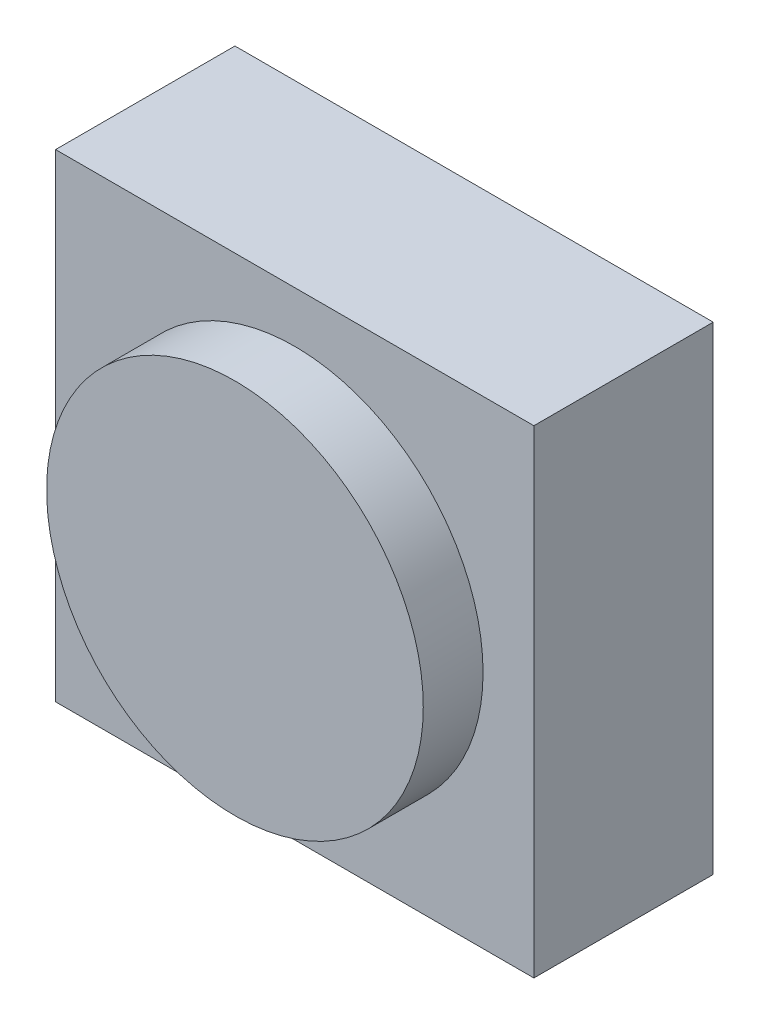
from build123d import *

# Parameters (mm, degrees)
SKETCH_1_W      = 80
SKETCH_1_H      = 80
EXTRUDE_1_DEPTH = 30
SKETCH_2_R      = 31.5
EXTRUDE_2_DEPTH = 10


with BuildPart() as part:
    # 草图1 → 凸台-拉伸1 (new body)
    with BuildSketch(Plane.XY):
        Rectangle(SKETCH_1_W, SKETCH_1_H)
    extrude(amount=EXTRUDE_1_DEPTH)

    # 草图2 → 凸台-拉伸2 (add)
    with BuildSketch(Plane.XY.offset(30)):
        Circle(SKETCH_2_R)
    extrude(amount=EXTRUDE_2_DEPTH)


solid = part.part
